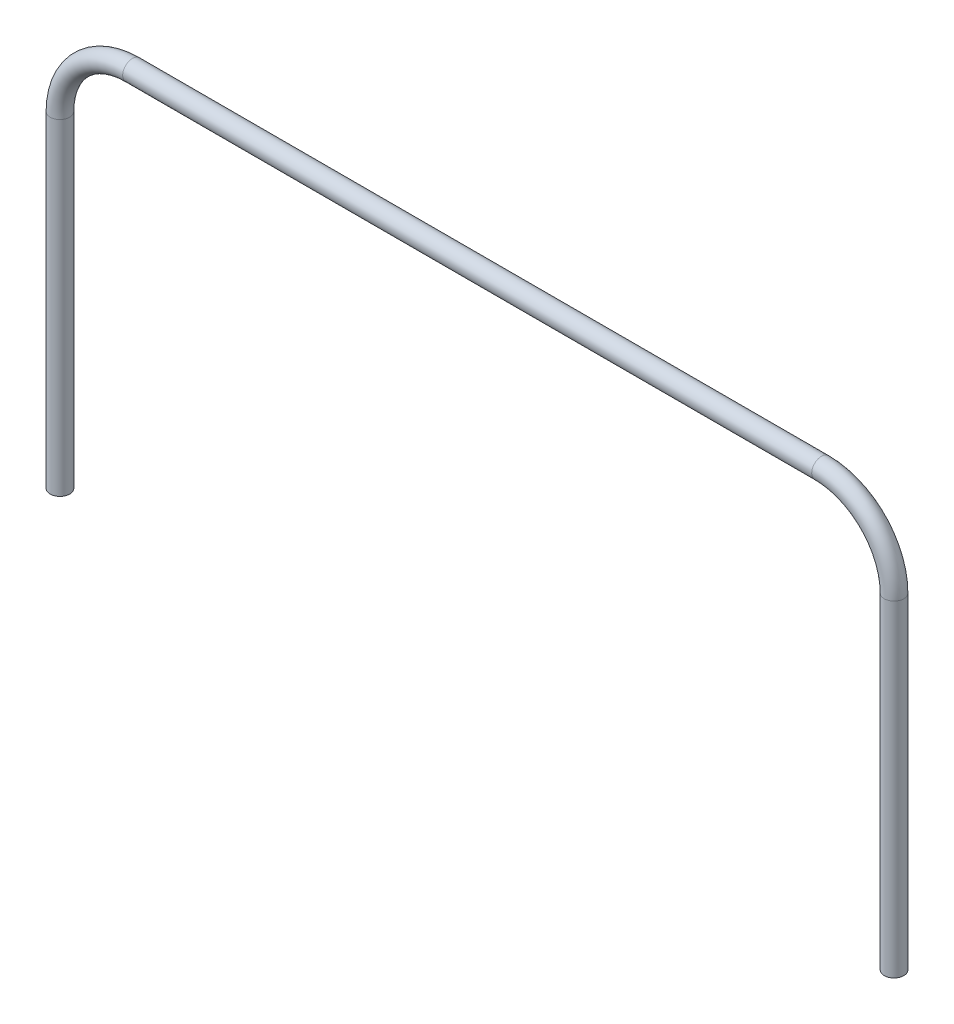
from build123d import *

# Parameters (mm, degrees)
SWEEP_1_PROFILE_R   = 13.5
SWEEP_1_PROFILE_R_2 = 12.5


with BuildPart() as part:
    # 扫描-薄件1: sweep along a path in 草图1
    with BuildLine(Plane.XY) as sweep_1_path:
        Line((-575, 0), (-575, 450))
        ThreePointArc((-575, 450), (-545.710678119, 520.710678119), (-475, 550))
        Line((-475, 550), (475, 550))
        ThreePointArc((475, 550), (545.710678119, 520.710678119), (575, 450))
        Line((575, 450), (575, 0))
    # 扫描-薄件1 profile (on start of the path) → 扫描-薄件1 (sweep)
    with BuildSketch(Plane(origin=(-575, 0, 0), x_dir=(0, 0, 1), z_dir=(0, 1, 0))):
        Circle(SWEEP_1_PROFILE_R)
        Circle(SWEEP_1_PROFILE_R_2, mode=Mode.SUBTRACT)
    sweep(path=sweep_1_path.line)


solid = part.part
